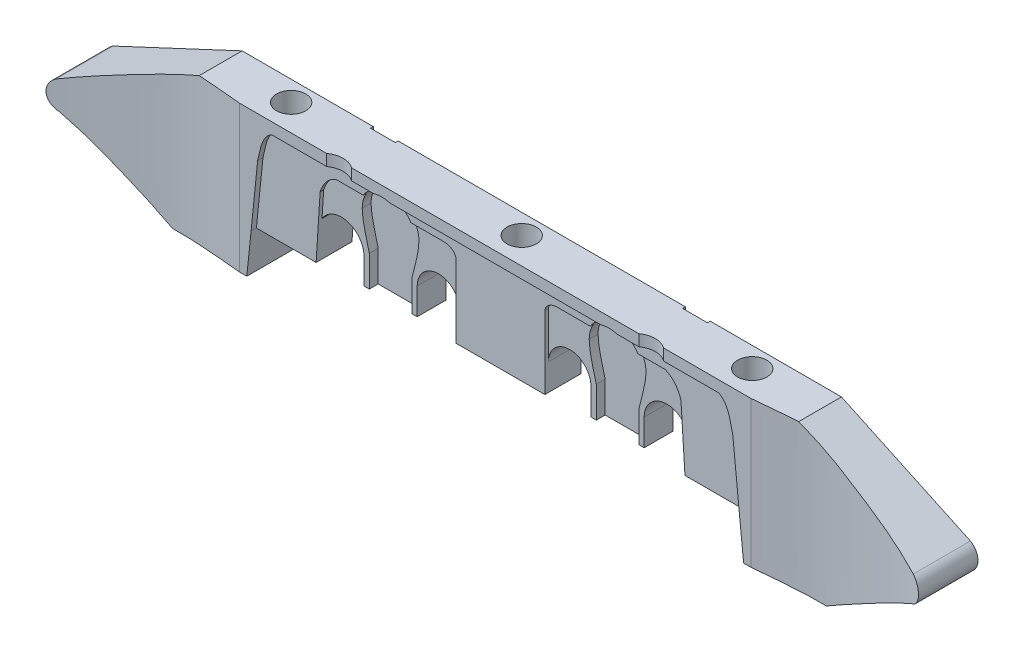
from build123d import *
from build123d.topology import SkipClean

# Parameters (mm, degrees)
EXTRUDE_1_DEPTH        = 165
SKETCH_2_R             = 16.5
CUT_EXTRUDE_1_DEPTH    = 25
SKETCH_3_R             = 12.5
CUT_EXTRUDE_2_DEPTH    = 50
SKETCH_4_R             = 5
CUT_EXTRUDE_3_DEPTH    = 1002.002622496
CUT_EXTRUDE_4_DEPTH    = 1002.002622496
CUT_EXTRUDE_6_DEPTH    = 26.25
CUT_EXTRUDE_17_DEPTH   = 6
CUT_EXTRUDE_18_DEPTH   = 10
MIRROR_9_COPY_1_DEPTH  = 26.25
MIRROR_9_COPY_2_DEPTH  = 26.25
MIRROR_11_COPY_1_DEPTH = 6
MIRROR_11_COPY_2_DEPTH = 10
CUT_EXTRUDE_19_DEPTH   = 1000.119946489
CUT_EXTRUDE_20_DEPTH   = 20
MIRROR_13_COPY_1_DEPTH = 20


with BuildPart() as part:
    # 草图1 → 凸台-拉伸1 (new body)
    with BuildSketch(Plane(origin=(0, 0, 0), x_dir=(1, 0, 0), z_dir=(0, 1, 0))):
        with BuildLine():
            Line((492, 0), (492, -52.5))
            Line((492, -52.5), (330, -52.5))
            ThreePointArc((330, -52.5), (316, -47.952239117), (302, -52.5))
            Line((302, -52.5), (203.688947417, -52.5))
            add(Edge.make_bspline(
                [(-1, -67.5), (16.270397527, -61.570196594), (46.073821795, -55.035068963), (86.891748272, -50.446322701), (137.401770931, -45.503584307), (176.084237464, -50.073931212), (203.688947417, -52.5)],
                knots=[0, 0, 0, 0, 0.264704673, 0.440851873, 0.596045826, 1, 1, 1, 1], degree=3))
            Line((-1, -67.5), (-1, -52.5))
            Line((-1, -52.5), (0, 0))
            Line((0, 0), (302, 0))
            Line((302, 0), (302, -3.15))
            Line((302, -3.15), (330, -3.15))
            Line((330, -3.15), (330, 0))
            Line((330, 0), (492, 0))
        make_face()
    extrude_1 = extrude(amount=-EXTRUDE_1_DEPTH)

    # 镜向2: 凸台-拉伸1 across plane
    add(extrude_1.mirror(Plane(origin=(492, -165, 0), x_dir=(0, 0, 1), z_dir=(1, 0, 0))))

    # 草图2 → 切除-拉伸1 (cut)
    with BuildSketch(Plane(origin=(0, 0, 0), x_dir=(1, 0, 0), z_dir=(0, 1, 0))):
        with Locations(Location((232, -22.63, 0), (0, 0, 270))):
            Circle(SKETCH_2_R)
        with BuildLine():
            Line((492, -6.13), (492, -39.13))
            ThreePointArc((492, -39.13), (475.5, -22.63), (492, -6.13))
        make_face()
    cut_extrude_1 = extrude(amount=-CUT_EXTRUDE_1_DEPTH, mode=Mode.SUBTRACT)

    # 镜向3: 切除-拉伸1 across plane
    with SkipClean():  # the faces are left unmerged after this step: merging them gives an invalid solid
        add(cut_extrude_1.mirror(Plane(origin=(492, 0, 0), x_dir=(0, 0, 1), z_dir=(1, 0, 0))), mode=Mode.SUBTRACT)

    # 草图3 → 切除-拉伸2 (cut)
    with SkipClean():  # the faces are left unmerged after this step: merging them gives an invalid solid
        with BuildSketch(Plane(origin=(0, 0, 0), x_dir=(1, 0, 0), z_dir=(0, 1, 0))):
            with Locations(Location((232, -22.63, 0), (0, 0, 270))):
                Circle(SKETCH_3_R)
            with BuildLine():
                Line((492, -10.13), (492, -35.13))
                ThreePointArc((492, -35.13), (479.5, -22.63), (492, -10.13))
            make_face()
        cut_extrude_2 = extrude(amount=-CUT_EXTRUDE_2_DEPTH, mode=Mode.SUBTRACT)

    # 草图4 → 切除-拉伸3 (cut, through all)
    with SkipClean():  # the faces are left unmerged after this step: merging them gives an invalid solid
        with BuildSketch(Plane(origin=(0, 0, 0), x_dir=(1, 0, 0), z_dir=(0, 1, 0))):
            with Locations(Location((232, -22.63, 0), (0, 0, 270))):
                Circle(SKETCH_4_R)
            with BuildLine():
                Line((492, -17.63), (492, -27.63))
                ThreePointArc((492, -27.63), (487, -22.63), (492, -17.63))
            make_face()
        cut_extrude_3 = extrude(amount=-CUT_EXTRUDE_3_DEPTH, mode=Mode.SUBTRACT)

    # 镜向4: 切除-拉伸2, 切除-拉伸3 across plane
    with SkipClean():  # the faces are left unmerged after this step: merging them gives an invalid solid
        add(cut_extrude_2.mirror(Plane(origin=(492, 0, 0), x_dir=(0, 0, 1), z_dir=(1, 0, 0))), mode=Mode.SUBTRACT)
        add(cut_extrude_3.mirror(Plane(origin=(492, 0, 0), x_dir=(0, 0, 1), z_dir=(1, 0, 0))), mode=Mode.SUBTRACT)

    # 草图5 → 切除-拉伸4 (cut, through all)
    with SkipClean():  # the faces are left unmerged after this step: merging them gives an invalid solid
        with BuildSketch(Plane(origin=(0, 0, 0), x_dir=(-1, 0, 0), z_dir=(0, 0, -1))):
            with BuildLine():
                Line((-985, 0), (-830, 0))
                Line((-830, 0), (-975.026271995, -67.813179655))
                Line((-975.026271995, -67.813179655), (-975.427385117, -68.000737094))
                ThreePointArc((-975.427385117, -68.000737094), (-981.640882236, -74.110927527), (-984, -82.5))
                ThreePointArc((-984, -82.5), (-981.027354106, -92.336692453), (-972.920433051, -98.651355789))
                Line((-972.920433051, -98.651355789), (-860.667769742, -165))
                Line((-860.667769742, -165), (-985, -165))
                Line((-985, -165), (-985, 0))
            make_face()
        cut_extrude_4 = extrude(amount=-CUT_EXTRUDE_4_DEPTH, mode=Mode.SUBTRACT)

    # 草图7 → 切除-拉伸6 (cut)
    with SkipClean():  # the faces are left unmerged after this step: merging them gives an invalid solid
        with BuildSketch(Plane.XY.offset(52.5)):
            Polygon((492, -118.447924154), (492, -165), (772.181034773, -165), (767.332212432, -118.447924154), align=None)
        cut_extrude_6 = extrude(amount=-CUT_EXTRUDE_6_DEPTH, mode=Mode.SUBTRACT)

    # 镜向6: 切除-拉伸6 across plane
    with SkipClean():  # the faces are left unmerged after this step: merging them gives an invalid solid
        add(cut_extrude_6.mirror(Plane.XY.offset(26.25)), mode=Mode.SUBTRACT)

    # 草图12 → 切除-拉伸17 (cut)
    with SkipClean():  # the faces are left unmerged after this step: merging them gives an invalid solid
        with BuildSketch(Plane.XY.offset(52.5)):
            with BuildLine():
                Line((492, -12.75914724), (744.10361322, -12.75914724))
                add(Edge.make_bspline(
                    [(744.10361322, -12.75914724), (748.90160638, -15.259093113), (756.502673834, -26.061308146), (758.103898877, -38.864285497), (759.933879657, -45.970617486)],
                    knots=[0, 0, 0, 0, 0.415607433, 1, 1, 1, 1], degree=3))
                Line((759.933879657, -45.970617486), (767.332212432, -118.447924154))
                Line((767.332212432, -118.447924154), (492, -118.447924154))
                Line((492, -118.447924154), (492, -12.75914724))
            make_face()
        cut_extrude_17 = extrude(amount=-CUT_EXTRUDE_17_DEPTH, mode=Mode.SUBTRACT)

    # 草图22 → 切除-拉伸18 (cut)
    with SkipClean():  # the faces are left unmerged after this step: merging them gives an invalid solid
        with BuildSketch(Plane.XY.offset(52.5)):
            with BuildLine():
                Line((542, -118.447924154), (700, -118.447924154))
                Line((700, -118.447924154), (695.482225258, -47.238610738))
                add(Edge.make_bspline(
                    [(677.168822524, -26.10759763), (686.656293957, -29.142996692), (692.738801615, -38.148785109), (695.482225258, -47.238610738)],
                    knots=[0, 0, 0, 0, 1, 1, 1, 1], degree=3))
                Line((677.168822524, -26.10759763), (555.906825709, -26.10759763))
                add(Edge.make_bspline(
                    [(542, -36.447924154), (542.796201016, -29.754247305), (549.823270443, -26.072180854), (555.906825709, -26.10759763)],
                    knots=[0, 0, 0, 0, 1, 1, 1, 1], degree=3))
                Line((542, -36.447924154), (542, -118.447924154))
            make_face()
        cut_extrude_18 = extrude(amount=-CUT_EXTRUDE_18_DEPTH, mode=Mode.SUBTRACT)

    # 镜向7: 切除-拉伸4 across plane
    with SkipClean():  # the faces are left unmerged after this step: merging them gives an invalid solid
        add(cut_extrude_4.mirror(Plane(origin=(492, 0, 0), x_dir=(0, 0, 1), z_dir=(1, 0, 0))), mode=Mode.SUBTRACT)

    # 镜向8: 切除-拉伸6 across plane
    with SkipClean():  # the faces are left unmerged after this step: merging them gives an invalid solid
        add(cut_extrude_6.mirror(Plane(origin=(492, 0, 0), x_dir=(0, 0, 1), z_dir=(1, 0, 0))), mode=Mode.SUBTRACT)

    # 镜向9 copy 1 sketch → 镜向9 copy 1 (cut)
    with BuildSketch(Plane(origin=(984, 0, 0), x_dir=(-1, 0, 0), z_dir=(0, 0, -1))):
        Polygon((492, -118.447924154), (492, -165), (772.181034773, -165), (767.332212432, -118.447924154), align=None)
    extrude(amount=-MIRROR_9_COPY_1_DEPTH, mode=Mode.SUBTRACT)

    # 镜向9 copy 2 sketch → 镜向9 copy 2 (cut)
    with BuildSketch(Plane(origin=(0, 0, 0), x_dir=(1, 0, 0), z_dir=(0, 0, -1))):
        Polygon((492, 118.447924154), (492, 165), (772.181034773, 165), (767.332212432, 118.447924154), align=None)
    extrude(amount=-MIRROR_9_COPY_2_DEPTH, mode=Mode.SUBTRACT)

    # 镜向10: 切除-拉伸17, 切除-拉伸18 across plane
    add(cut_extrude_17.mirror(Plane(origin=(492, 0, 0), x_dir=(0, 0, 1), z_dir=(1, 0, 0))), mode=Mode.SUBTRACT)
    add(cut_extrude_18.mirror(Plane(origin=(492, 0, 0), x_dir=(0, 0, 1), z_dir=(1, 0, 0))), mode=Mode.SUBTRACT)

    # 镜向11: 切除-拉伸17, 切除-拉伸18 across plane
    add(cut_extrude_17.mirror(Plane.XY.offset(26.25)), mode=Mode.SUBTRACT)
    add(cut_extrude_18.mirror(Plane.XY.offset(26.25)), mode=Mode.SUBTRACT)

    # 镜向11 copy 1 sketch → 镜向11 copy 1 (cut)
    with BuildSketch(Plane(origin=(984, 0, 0), x_dir=(-1, 0, 0), z_dir=(0, 0, -1))):
        with BuildLine():
            Line((492, -12.75914724), (744.10361322, -12.75914724))
            add(Edge.make_bspline(
                [(744.10361322, -12.75914724), (748.90160638, -15.259093113), (756.502673834, -26.061308146), (758.103898877, -38.864285497), (759.933879657, -45.970617486)],
                knots=[0, 0, 0, 0, 0.415607433, 1, 1, 1, 1], degree=3))
            Line((759.933879657, -45.970617486), (767.332212432, -118.447924154))
            Line((767.332212432, -118.447924154), (492, -118.447924154))
            Line((492, -118.447924154), (492, -12.75914724))
        make_face()
    extrude(amount=-MIRROR_11_COPY_1_DEPTH, mode=Mode.SUBTRACT)

    # 镜向11 copy 2 sketch → 镜向11 copy 2 (cut)
    with BuildSketch(Plane(origin=(984, 0, 0), x_dir=(-1, 0, 0), z_dir=(0, 0, -1))):
        with BuildLine():
            Line((542, -118.447924154), (700, -118.447924154))
            Line((700, -118.447924154), (695.482225258, -47.238610738))
            add(Edge.make_bspline(
                [(677.168822524, -26.10759763), (686.656293957, -29.142996692), (692.738801615, -38.148785109), (695.482225258, -47.238610738)],
                knots=[0, 0, 0, 0, 1, 1, 1, 1], degree=3))
            Line((677.168822524, -26.10759763), (555.906825709, -26.10759763))
            add(Edge.make_bspline(
                [(542, -36.447924154), (542.796201016, -29.754247305), (549.823270443, -26.072180854), (555.906825709, -26.10759763)],
                knots=[0, 0, 0, 0, 1, 1, 1, 1], degree=3))
            Line((542, -36.447924154), (542, -118.447924154))
        make_face()
    extrude(amount=-MIRROR_11_COPY_2_DEPTH, mode=Mode.SUBTRACT)

    # 草图23 → 切除-拉伸19 (cut, through all)
    with BuildSketch(Plane.XY.offset(52.5)):
        with BuildLine():
            Line((442, -118.447924154), (394, -118.447924154))
            Line((394, -118.447924154), (394, -88.447924154))
            ThreePointArc((394, -88.447924154), (418, -64.447924154), (442, -88.447924154))
            Line((442, -88.447924154), (442, -118.447924154))
        make_face()
        with BuildLine():
            Line((590, -118.447924154), (590, -88.447924154))
            ThreePointArc((590, -88.447924154), (566, -64.447924154), (542, -88.447924154))
            Line((542, -88.447924154), (542, -118.447924154))
            Line((542, -118.447924154), (590, -118.447924154))
        make_face()
        with BuildLine():
            Line((650, -118.447924154), (700, -118.447924154))
            Line((700, -118.447924154), (697.252435673, -75.140725265))
            ThreePointArc((697.252435673, -75.140725265), (668.587587602, -63.902689284), (650, -88.447924154))
            Line((650, -88.447924154), (650, -118.447924154))
        make_face()
        with BuildLine():
            Line((334, -118.447924154), (284, -118.447924154))
            Line((284, -118.447924154), (286.682338557, -76.168815981))
            ThreePointArc((286.682338557, -76.168815981), (314.920895332, -64.660351674), (334, -88.447924154))
            Line((334, -88.447924154), (334, -118.447924154))
        make_face()
    extrude(amount=-CUT_EXTRUDE_19_DEPTH, mode=Mode.SUBTRACT)

    # 草图24 → 切除-拉伸20 (cut)
    with BuildSketch(Plane.XY.offset(52.5)):
        with BuildLine():
            Line((620, -118.447924154), (644, -118.447924154))
            Line((644, -118.447924154), (644, -83.447924154))
            add(Edge.make_bspline(
                [(652, -43.395707029), (651.638960409, -57.163414003), (647.108632556, -70.19764028), (644, -83.447924154)],
                knots=[0, 0, 0, 0, 1, 1, 1, 1], degree=3))
            ThreePointArc((652, -43.395707029), (620, -11.395707029), (588, -43.395707029))
            add(Edge.make_bspline(
                [(588, -43.395707029), (588.361039599, -57.163414002), (592.891367445, -70.197640279), (596, -83.447924154)],
                knots=[0, 0, 0, 0, 1, 1, 1, 1], degree=3))
            Line((596, -83.447924154), (596, -118.447924154))
            Line((596, -118.447924154), (620, -118.447924154))
        make_face()
    cut_extrude_20 = extrude(amount=-CUT_EXTRUDE_20_DEPTH, mode=Mode.SUBTRACT)

    # 镜向12: 切除-拉伸20 across plane
    add(cut_extrude_20.mirror(Plane(origin=(492, 0, 0), x_dir=(0, 0, 1), z_dir=(1, 0, 0))), mode=Mode.SUBTRACT)

    # 镜向13: 切除-拉伸20 across plane
    add(cut_extrude_20.mirror(Plane.XY.offset(26.25)), mode=Mode.SUBTRACT)

    # 镜向13 copy 1 sketch → 镜向13 copy 1 (cut)
    with BuildSketch(Plane(origin=(984, 0, 0), x_dir=(-1, 0, 0), z_dir=(0, 0, -1))):
        with BuildLine():
            Line((620, -118.447924154), (644, -118.447924154))
            Line((644, -118.447924154), (644, -83.447924154))
            add(Edge.make_bspline(
                [(652, -43.395707029), (651.638960409, -57.163414003), (647.108632556, -70.19764028), (644, -83.447924154)],
                knots=[0, 0, 0, 0, 1, 1, 1, 1], degree=3))
            ThreePointArc((652, -43.395707029), (620, -11.395707029), (588, -43.395707029))
            add(Edge.make_bspline(
                [(588, -43.395707029), (588.361039599, -57.163414002), (592.891367445, -70.197640279), (596, -83.447924154)],
                knots=[0, 0, 0, 0, 1, 1, 1, 1], degree=3))
            Line((596, -83.447924154), (596, -118.447924154))
            Line((596, -118.447924154), (620, -118.447924154))
        make_face()
    extrude(amount=-MIRROR_13_COPY_1_DEPTH, mode=Mode.SUBTRACT)


solid = part.part
